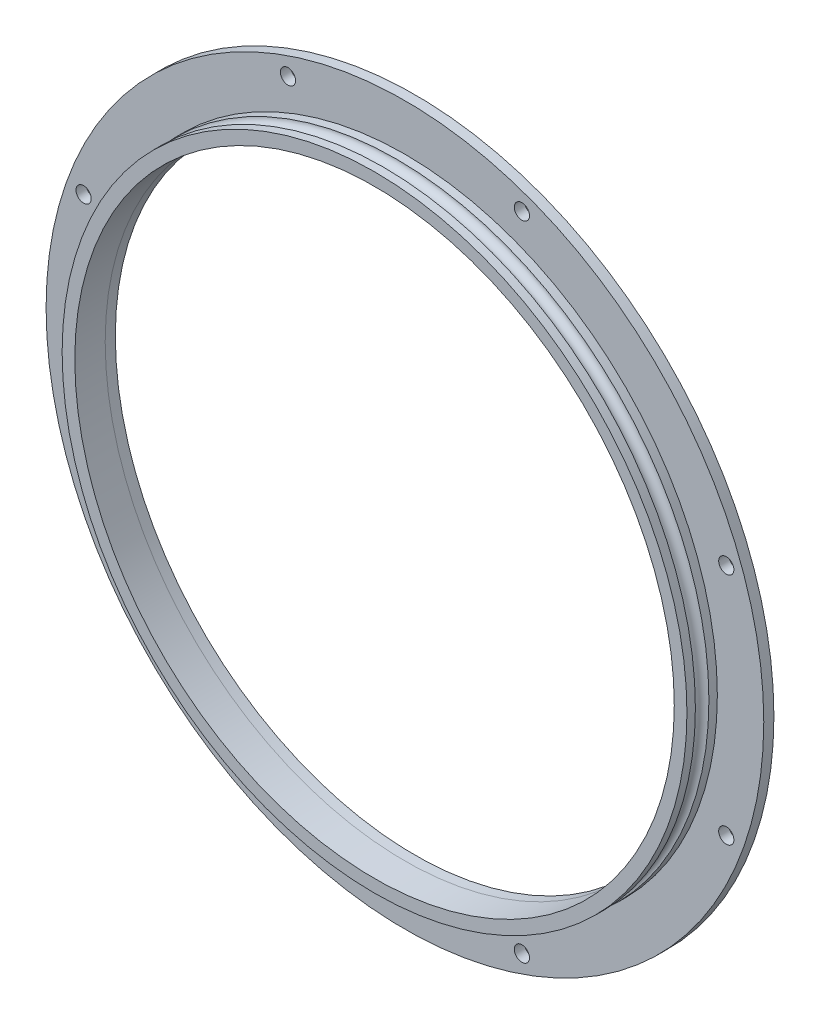
from build123d import *

# Parameters (mm, degrees)
SKETCH_1_R          = 425
SKETCH_1_R_2        = 355
EXTRUDE_1_DEPTH     = 12
SKETCH_2_R          = 370
SKETCH_2_R_2        = 355
EXTRUDE_2_DEPTH     = 36
SWEEP_1_PROFILE_R   = 8
SKETCH_12_R         = 9
CUT_EXTRUDE_1_DEPTH = 20


with BuildPart() as part:
    # 草图1 → 凸台-拉伸1 (new body)
    with BuildSketch(Plane.XY):
        Circle(SKETCH_1_R)
        Circle(SKETCH_1_R_2, mode=Mode.SUBTRACT)
    extrude(amount=EXTRUDE_1_DEPTH)

    # 草图12 → 切除-拉伸1 (cut)
    with BuildSketch(Plane.XY.offset(12)):
        with Locations((-138.5, 380.582119916)):
            Circle(SKETCH_12_R)
        with Locations((138.5, 380.582119916)):
            Circle(SKETCH_12_R)
        with Locations((138.5, -380.582119916)):
            Circle(SKETCH_12_R)
        with Locations((-138.5, -380.582119916)):
            Circle(SKETCH_12_R)
        with Locations((-380.582119916, 138.5)):
            Circle(SKETCH_12_R)
        with Locations((-380.582119916, -138.5)):
            Circle(SKETCH_12_R)
        with Locations((380.582119916, -138.5)):
            Circle(SKETCH_12_R)
        with Locations((380.582119916, 138.5)):
            Circle(SKETCH_12_R)
    extrude(amount=-CUT_EXTRUDE_1_DEPTH, mode=Mode.SUBTRACT)


with BuildPart() as body_2:
    # 草图2 → 凸台-拉伸2 (new body)
    with BuildSketch(Plane.XY.offset(12)):
        Circle(SKETCH_2_R)
        Circle(SKETCH_2_R_2, mode=Mode.SUBTRACT)
    extrude(amount=EXTRUDE_2_DEPTH)

    # 切除-扫描1: sweep along a path in 草图3
    with BuildLine(Plane(origin=(0, 0, 30), x_dir=(-1, 0, 0), z_dir=(0, 0, -1))) as sweep_1_path:
        CenterArc((0, 0), 370, 0, 360)
    # 切除-扫描1 profile (on start of the path) → 切除-扫描1 (sweep, cut)
    with BuildSketch(Plane(origin=(-370, 0, 30), x_dir=(0, 0, 1), z_dir=(0, 1, 0))):
        Circle(SWEEP_1_PROFILE_R)
    sweep(path=sweep_1_path.line, mode=Mode.SUBTRACT)


solid = Compound([part.part, body_2.part])
